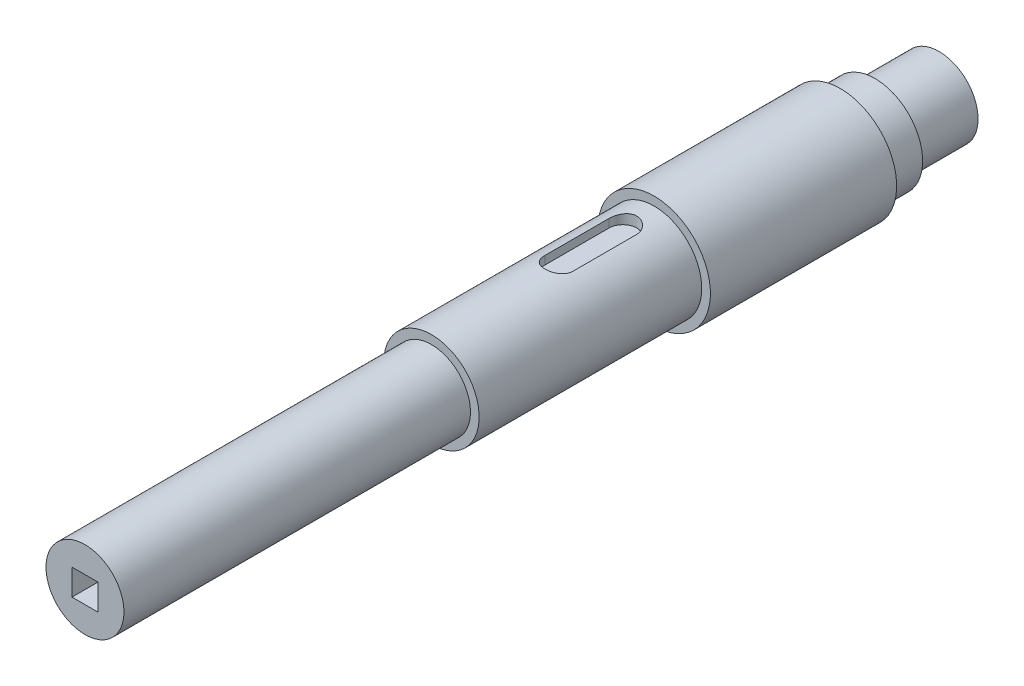
from build123d import *

# Parameters (mm, degrees)
SKETCH_2_W          = 15
SKETCH_2_H          = 15
CUT_EXTRUDE_1_DEPTH = 496.137859591
CHAMFER_1_SIZE      = 3
CHAMFER_1_SIZE2     = 5.196152423
CUT_EXTRUDE_2_DEPTH = 6


with BuildPart() as part:
    # 草图1 → 旋转1 (revolve)
    with BuildSketch(Plane(origin=(0, 0, 0), x_dir=(1, 0, 0), z_dir=(0, 1, 0))):
        Polygon((0, 200), (-22.5, 200), (-22.5, 163), (-27.5, 163), (-27.5, 143), (-32.5, 143), (-32.5, 35.5), (-27.5, 35.5), (-27.5, -93), (-22.5, -93), (-22.5, -293), (0, -293), align=None)
    revolve(axis=Axis((0, 0, 0), (0, 0, 1)))

    # 草图2 → 切除-拉伸1 (cut, through all)
    with BuildSketch(Plane(origin=(0, 0, -200), x_dir=(-1, 0, 0), z_dir=(0, 0, -1))):
        Rectangle(SKETCH_2_W, SKETCH_2_H)
    extrude(amount=-CUT_EXTRUDE_1_DEPTH, mode=Mode.SUBTRACT)

    # 倒角1
    chamfer_1_edges = [part.edges().sort_by_distance(p)[0] for p in [
        (7.5, 0, -200),
        (0, -7.5, -200),
        (-7.5, 0, -200),
        (0, 7.5, -200),
    ]]
    chamfer_1_side = [part.faces().sort_by_distance(p)[0] for p in [
        (21.863603897, 0, -200),
    ]]
    chamfer(chamfer_1_edges, length=CHAMFER_1_SIZE, length2=CHAMFER_1_SIZE2, reference=chamfer_1_side[0])

    # 草图3 → 切除-拉伸2 (cut)
    with BuildSketch(Plane(origin=(0, 27.5, 0), x_dir=(1, 0, 0), z_dir=(0, 1, 0))):
        with BuildLine():
            Line((-8, -19.5), (-8, 17.5))
            ThreePointArc((-8, 17.5), (0, 25.5), (8, 17.5))
            Line((8, 17.5), (8, -19.5))
            ThreePointArc((8, -19.5), (0, -27.5), (-8, -19.5))
        make_face()
    extrude(amount=-CUT_EXTRUDE_2_DEPTH, mode=Mode.SUBTRACT)


solid = part.part
